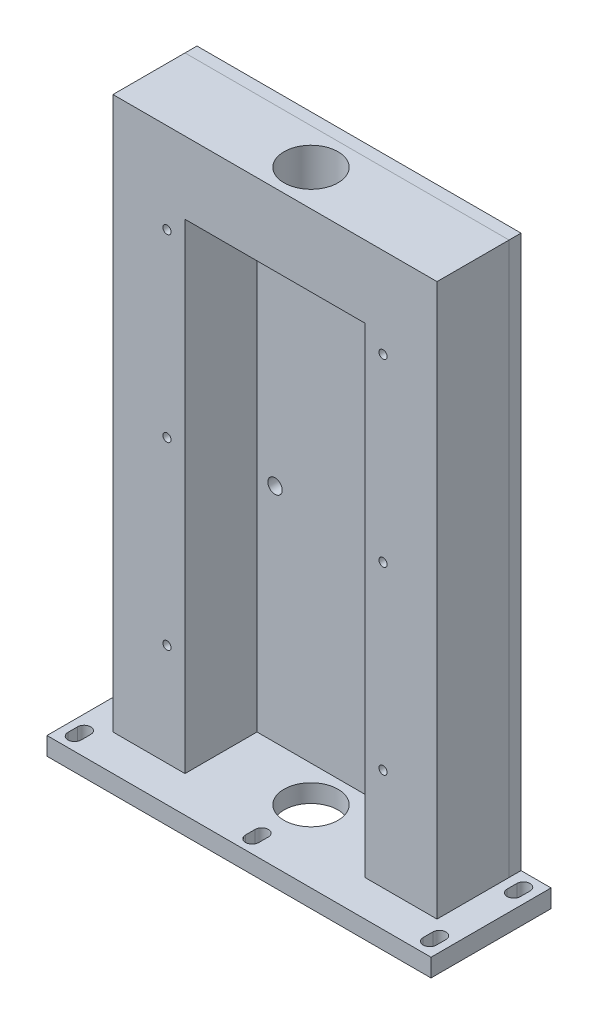
SolidWorks part; units mm, degrees
ref_plane "Front Plane" through (0, 0, 0) normal (0, 0, 1) x (1, 0, 0)
ref_plane "Top Plane" through (0, 0, 0) normal (0, 1, 0) x (1, 0, 0)
ref_plane "Right Plane" through (0, 0, 0) normal (1, 0, 0) x (0, 0, -1)
sketch "Sketch1" plane through (0, 0, 0) normal (0, 0, 1) x (1, 0, 0)
  line L0 (0, 0) -> (138.2504, 0) construction
  line L1 (-135, 460) -> (135, 460)
  line L2 (-135, 460) -> (-135, 0)
  line L3 (-135, 0) -> (-75, 0)
  line L4 (-75, 400) -> (-75, 0)
  line L5 (0, 0) -> (0, 197.8382) construction
  line L6 (75, 400) -> (75, 0)
  line L7 (135, 0) -> (75, 0)
  line L8 (135, 460) -> (135, 0)
  line L13 (-75, 400) -> (75, 400)
  dimension "D1" = 150
  dimension "D2" = 460
  dimension "D3" = 135
  dimension "D4" = 60
extrude "Boss-Extrude1" add sketch "Sketch1" along normal blind 60
sketch "Sketch3" plane through (0, 0, 0) normal (0, 0, -1) x (-1, 0, 0)
  line L1 (-135, 460) -> (135, 460)
  line L2 (-135, 460) -> (-135, 0)
  line L3 (-135, 0) -> (135, 0)
  line L4 (135, 460) -> (135, 0)
extrude "Boss-Extrude3" add sketch "Sketch3" along normal blind 10 separate body
sketch "Sketch4" plane through (0, 0, 0) normal (0, -1, 0) x (1, 0, 0)
  line L1 (135, -10) -> (-135, -10) construction
  line L2 (-160, 90) -> (160, 90)
  line L3 (-160, 90) -> (-160, -10)
  line L4 (-160, -10) -> (160, -10)
  line L5 (160, 90) -> (160, -10)
  line L7 (0, 0) -> (0, 88.2378) construction
  dimension "D1" = 320
  dimension "D2" = 100
extrude "Boss-Extrude4" add sketch "Sketch4" along normal blind 15 separate body
sketch "Sketch7" plane through (0, 0, 0) normal (0, 1, 0) x (1, 0, 0)
  line L0 (0, 0) -> (0, -125.5042) construction
  line L1 (160, -40) -> (221.9033, -40) construction
  line L2 (160, 10) -> (160, -90) construction
  line L3 (160, -90) -> (-160, -90) construction
  circle A0 centre (148, -5) radius 5.5
  circle A1 centre (148, -75) radius 5.5
  circle A2 centre (-148, -75) radius 5.5
  circle A3 centre (-148, -5) radius 5.5
  circle A4 centre (0, -75) radius 5.5
  dimension "D1" = 11
  dimension "D4" = 11
  dimension "D2" = 12
  dimension "D3" = 35
  dimension "D5" = 15
extrude "Cut-Extrude1" cut sketch "Sketch7" against normal through all
sketch "Sketch22" plane through (0, 0, 0) normal (0, 1, 0) x (1, 0, 0)
  line L0 (-148, -1) -> (-148, -9) construction
  line L1 (-142.5, -1) -> (-142.5, -9)
  line L2 (-153.5, -1) -> (-153.5, -9)
  line L3 (-148, -71) -> (-148, -79) construction
  line L4 (-142.5, -71) -> (-142.5, -79)
  line L5 (-153.5, -71) -> (-153.5, -79)
  line L6 (0, 0) -> (0, -52.4914) construction
  line L7 (148, -1) -> (148, -9) construction
  line L8 (142.5, -1) -> (142.5, -9)
  line L9 (153.5, -1) -> (153.5, -9)
  line L10 (148, -71) -> (148, -79) construction
  line L11 (142.5, -71) -> (142.5, -79)
  line L12 (153.5, -71) -> (153.5, -79)
  line L13 (0, -71) -> (0, -79) construction
  line L14 (5.5, -71) -> (5.5, -79)
  line L15 (-5.5, -71) -> (-5.5, -79)
  arc A0 (-142.5, -1) -> (-153.5, -1) centre (-148, -1) ccw
  arc A1 (-153.5, -9) -> (-142.5, -9) centre (-148, -9) ccw
  arc A2 (-142.5, -71) -> (-153.5, -71) centre (-148, -71) ccw
  arc A3 (-153.5, -79) -> (-142.5, -79) centre (-148, -79) ccw
  arc A4 (142.5, -1) -> (153.5, -1) centre (148, -1) cw
  arc A5 (153.5, -9) -> (142.5, -9) centre (148, -9) cw
  arc A6 (142.5, -71) -> (153.5, -71) centre (148, -71) cw
  arc A7 (153.5, -79) -> (142.5, -79) centre (148, -79) cw
  arc A8 (5.5, -71) -> (-5.5, -71) centre (0, -71) ccw
  arc A9 (-5.5, -79) -> (5.5, -79) centre (0, -79) ccw
  point P3 (-148, -5)
  point P10 (-148, -75)
  point P21 (148, -5)
  point P28 (148, -75)
  point P36 (0, -75)
  dimension "D1" = 8
  dimension "D2" = 11
extrude "Cut-Extrude3" cut sketch "Sketch22" against normal through all
sketch "Sketch23" plane through (0, 460, 0) normal (0, 1, 0) x (1, 0, 0)
  line L0 (160, -90) -> (-160, -90) construction
  line L1 (0, 0) -> (0, -111.3041) construction
  circle A0 centre (0, -30) radius 22.5
  dimension "D1" = 60
  dimension "D2" = 45
extrude "Cut-Extrude4" cut sketch "Sketch23" against normal through all
sketch "Sketch24" plane through (0, 0, -10) normal (0, 0, -1) x (-1, 0, 0)
  circle A0 centre (-60, 257) radius 15
  dimension "D1" = 30
extrude "Cut-Extrude5" cut sketch "Sketch24" against normal through all
hole_wizard "M8 Tapped Hole1" positions "Sketch28" profile "Sketch27" tap size "M8" standard "Iso" end condition through all
sketch "Sketch28" plane through (0, 0, -10) normal (0, 0, -1) x (-1, 0, 0)
  line L0 (160, -15) -> (-160, -15) construction
  line L1 (0, 0) -> (0, 454.9999) construction
  line L2 (-135, 0) -> (135, 0) construction
  point P0 (-90, 385)
  point P2 (90, 385)
  point P4 (-90, 235)
  point P6 (90, 235)
  point P8 (-90, 85)
  point P10 (90, 85)
  dimension "D1" = 150
  dimension "D2" = 150
  dimension "D3" = 100
  dimension "D4" = 180
sketch "Sketch27" plane through (90, 385, -10) normal (1, 0, 0) x (0, 1, 0)
  line L0 (0, 0) -> (0, 100)
  line L1 (0, 100) -> (3.4, 100)
  line L2 (3.4, 100) -> (3.4, 0)
  line L5 (3.4, 0) -> (0, 0)
  line L11 (0, -6.35) -> (0, 107.95) construction
  dimension "通孔螺纹孔钻头直径" = 6.8
  dimension "通孔螺纹孔钻头深度" = 100
cosmetic thread "Cosmetic Thread20" parameters "D2"=8
cosmetic thread "Cosmetic Thread21" parameters "D2"=8
cosmetic thread "Cosmetic Thread22" parameters "D2"=8
cosmetic thread "Cosmetic Thread23" parameters "D2"=8
cosmetic thread "Cosmetic Thread24" parameters "D2"=8
cosmetic thread "Cosmetic Thread25" parameters "D2"=8
sketch "Sketch29" plane through (0, 0, -10) normal (0, 0, -1) x (-1, 0, 0)
  line L0 (0, 0) -> (0, 297.3069) construction
  line L1 (160, -15) -> (-160, -15) construction
  circle A0 centre (-60, 185) radius 6
  circle A1 centre (60, 185) radius 6
  dimension "D1" = 12
  dimension "D3" = 200
  dimension "D2" = 120
extrude "Cut-Extrude6" cut sketch "Sketch29" against normal blind 10
